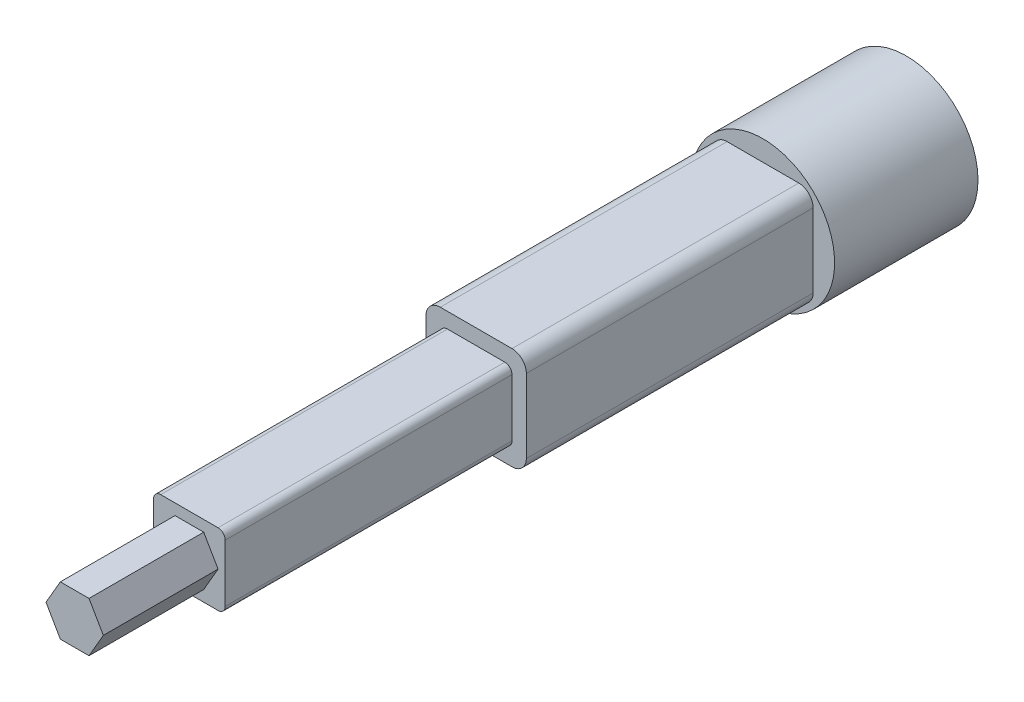
SolidWorks part; units mm, degrees
ref_plane "Front Plane" through (0, 0, 0) normal (0, 0, 1) x (1, 0, 0)
ref_plane "Top Plane" through (0, 0, 0) normal (0, 1, 0) x (1, 0, 0)
ref_plane "Right Plane" through (0, 0, 0) normal (1, 0, 0) x (0, 0, -1)
other "Configuration Table"
sketch "Sketch1" plane through (0, 0, 0) normal (0, 0, 1) x (1, 0, 0)
  circle A0 centre (0, 0) radius 5
  dimension "D1" = 10
extrude "Boss-Extrude1" add sketch "Sketch1" along normal blind 10
sketch "Sketch2" plane through (0, 0, 10) normal (0, 0, 1) x (1, 0, 0)
  line L1 (-3.5, 3.5707) -> (3.5, 3.5707)
  line L2 (-3.5, 3.5707) -> (-3.5, -3.5707)
  line L3 (-3.5, -3.5707) -> (3.5, -3.5707)
  line L4 (3.5, 3.5707) -> (3.5, -3.5707)
  circle A0 centre (0, 0) radius 5 construction
  dimension "D1" = 7
extrude "Boss-Extrude2" add sketch "Sketch2" along normal blind 20
fillet "Fillet1" radius 1 4 edges at (3.5, -3.5707, 20) (-3.5, -3.5707, 20) (-3.5, 3.5707, 20) (3.5, 3.5707, 20)
sketch "Sketch3" plane through (0, 0, 30) normal (0, 0, 1) x (1, 0, 0)
  line L1 (2.5, -2.5) -> (-2.5, -2.5)
  line L2 (2.5, -2.5) -> (2.5, 2.5)
  line L3 (2.5, 2.5) -> (-2.5, 2.5)
  line L4 (-2.5, -2.5) -> (-2.5, 2.5)
  line L5 (2.5, -2.5) -> (-2.5, 2.5) construction
  line L6 (2.5, 2.5) -> (-2.5, -2.5) construction
  point P0 (0, 0)
  dimension "D1" = 5
  dimension "D2" = 5
extrude "Boss-Extrude3" add sketch "Sketch3" along normal blind 20
fillet "Fillet2" radius 0.5 4 edges at (2.5, -2.5, 40) (-2.5, -2.5, 40) (-2.5, 2.5, 40) (2.5, 2.5, 40)
sketch "Sketch4" plane through (0, 0, 50) normal (0, 0, 1) x (1, 0, 0)
  line L1 (1, 1.7321) -> (-1, 1.7321)
  line L2 (-1, 1.7321) -> (-2, 0)
  line L3 (-2, 0) -> (-1, -1.7321)
  line L4 (-1, -1.7321) -> (1, -1.7321)
  line L5 (1, -1.7321) -> (2, 0)
  line L6 (2, 0) -> (1, 1.7321)
  circle A0 centre (0, 0) radius 1.7321 construction
  dimension "D1" = 2
extrude "Boss-Extrude4" add sketch "Sketch4" along normal blind 8
